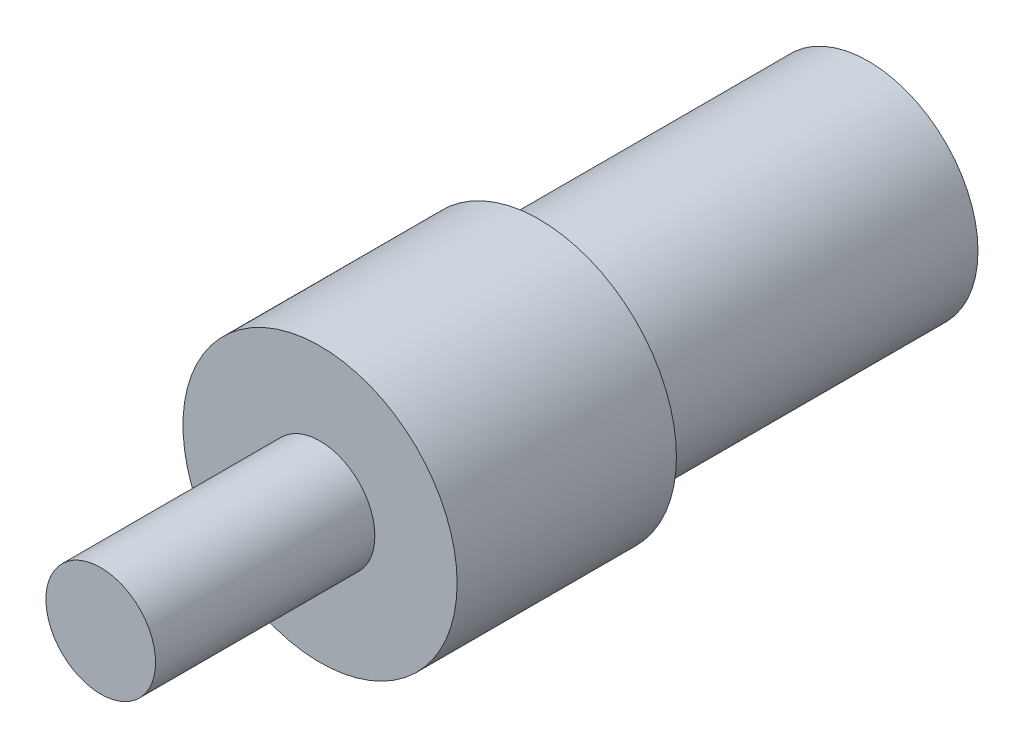
from build123d import *

# Parameters (mm, degrees)
SKETCH1_R           = 10
BOSS_EXTRUDE1_DEPTH = 30
SKETCH2_R           = 12.5
BOSS_EXTRUDE2_DEPTH = 20
SKETCH3_R           = 5
BOSS_EXTRUDE3_DEPTH = 20


with BuildPart() as part:
    # Sketch1 → Boss-Extrude1 (new body)
    with BuildSketch(Plane.XY):
        Circle(SKETCH1_R)
    extrude(amount=BOSS_EXTRUDE1_DEPTH)

    # Sketch2 → Boss-Extrude2 (add)
    with BuildSketch(Plane.XY.offset(30)):
        Circle(SKETCH2_R)
    extrude(amount=BOSS_EXTRUDE2_DEPTH)

    # Sketch3 → Boss-Extrude3 (add)
    with BuildSketch(Plane.XY.offset(50)):
        Circle(SKETCH3_R)
    extrude(amount=BOSS_EXTRUDE3_DEPTH)


solid = part.part
